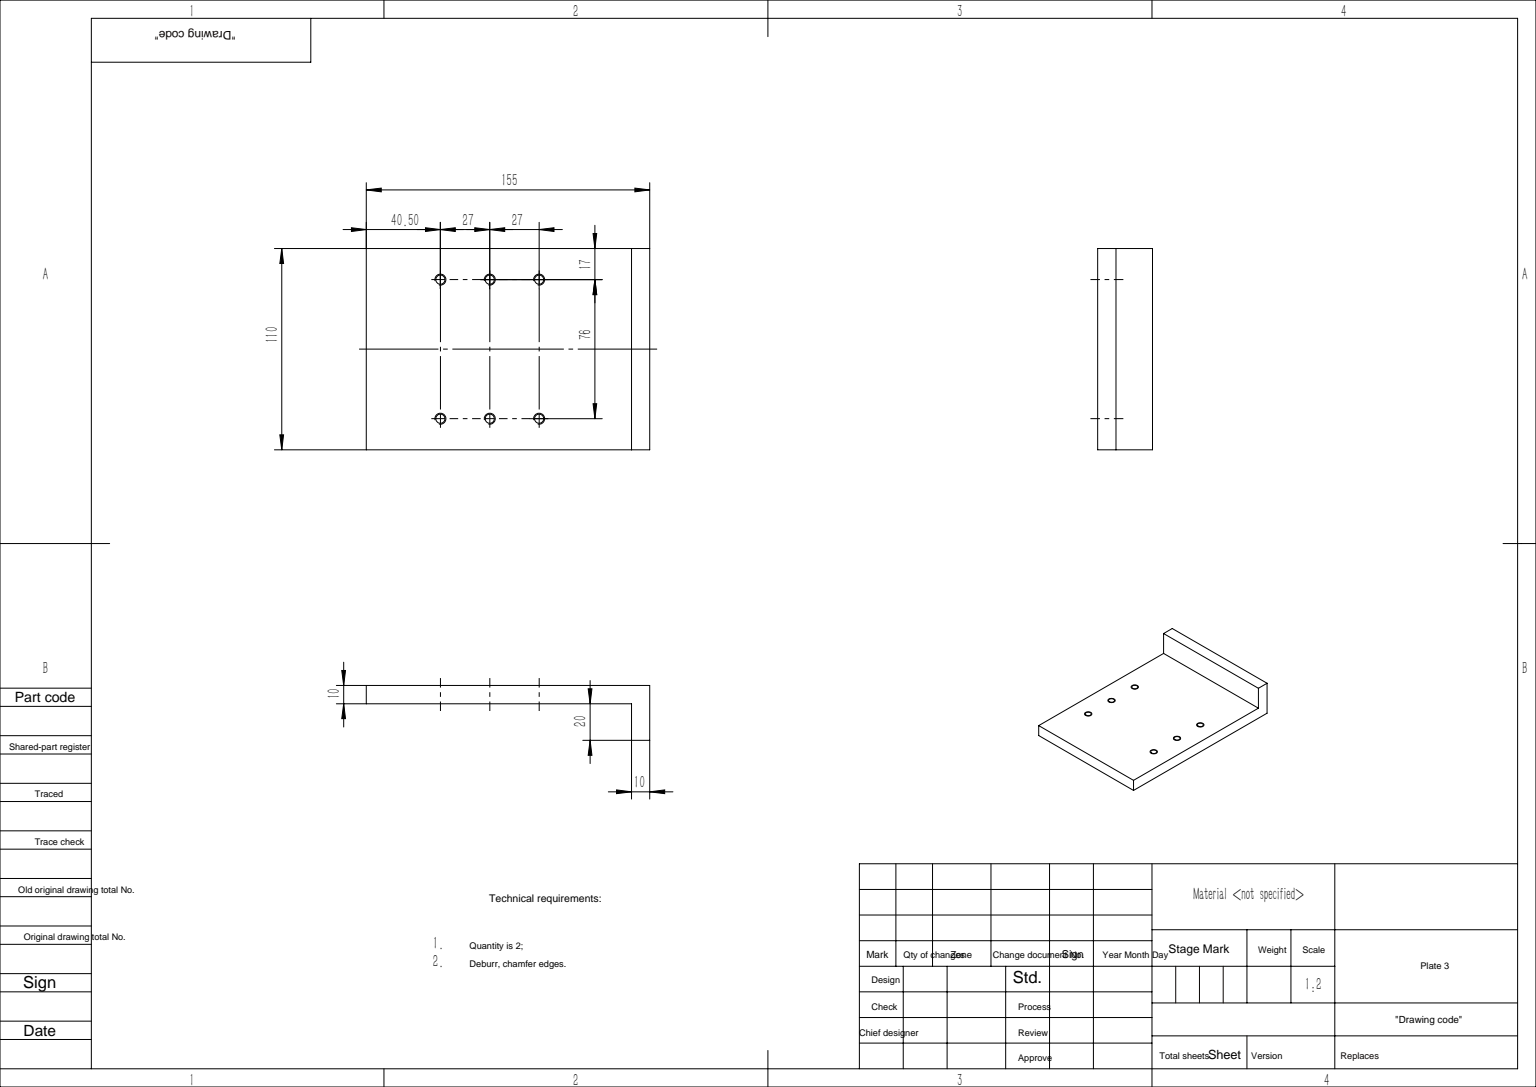
from build123d import *

# Parameters (mm, degrees)
SKETCH_2_W         = 110
SKETCH_2_H         = 135
EXTRUDE_1_DEPTH    = 10
HOLE_WIZARD_M6_1_D = 5
SKETCH_11_W        = 110
SKETCH_11_H        = 20
EXTRUDE_6_DEPTH    = 10
SKETCH_15_W        = 110
SKETCH_15_H        = 30
EXTRUDE_7_DEPTH    = 10


with BuildPart() as part:
    # 草图2 → 凸台-拉伸1 (new body)
    with BuildSketch(Plane(origin=(0, 0, 0), x_dir=(1, 0, 0), z_dir=(0, 1, 0))):
        Rectangle(SKETCH_2_W, SKETCH_2_H)
    extrude(amount=EXTRUDE_1_DEPTH)

    # M6 螺纹孔1 (through all)
    with Locations(Plane(origin=(0, 10, 0), x_dir=(1, 0, 0), z_dir=(0, 1, 0))):
        with Locations((-38, 27), (-38, 0), (38, 0), (-38, -27), (38, -27), (38, 27)):
            Hole(HOLE_WIZARD_M6_1_D / 2)

    # 草图11 → 凸台-拉伸6 (add)
    with BuildSketch(Plane.XZ):
        with Locations((0, -77.5)):
            Rectangle(SKETCH_11_W, SKETCH_11_H)
    extrude(amount=-EXTRUDE_6_DEPTH)

    # 草图15 → 凸台-拉伸7 (add)
    with BuildSketch(Plane(origin=(0, 0, -87.5), x_dir=(-1, 0, 0), z_dir=(0, 0, -1))):
        with Locations((0, 15)):
            Rectangle(SKETCH_15_W, SKETCH_15_H)
    extrude(amount=-EXTRUDE_7_DEPTH)


solid = part.part
